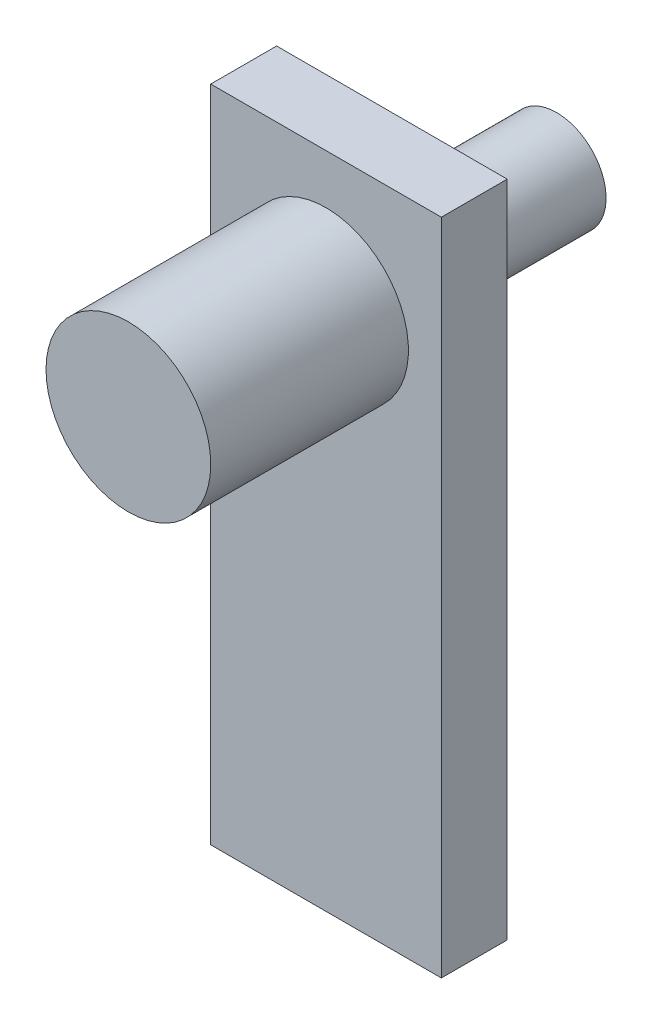
from build123d import *

# Parameters (mm, degrees)
SKETCH_1_W      = 35
SKETCH_1_H      = 100
EXTRUDE_1_DEPTH = 10
SKETCH_2_R      = 12.5
EXTRUDE_2_DEPTH = 30
SKETCH_3_R      = 7.5
EXTRUDE_3_DEPTH = 25


with BuildPart() as part:
    # 草图1 → 凸台-拉伸1 (new body)
    with BuildSketch(Plane.XY):
        Rectangle(SKETCH_1_W, SKETCH_1_H)
    extrude(amount=EXTRUDE_1_DEPTH)

    # 草图2 → 凸台-拉伸2 (add)
    with BuildSketch(Plane.XY.offset(10)):
        with Locations(Location((0, 30, 0), (0, 0, 180))):
            Circle(SKETCH_2_R)
    extrude(amount=EXTRUDE_2_DEPTH)

    # 草图3 → 凸台-拉伸3 (add)
    with BuildSketch(Plane(origin=(0, 0, 0), x_dir=(-1, 0, 0), z_dir=(0, 0, -1))):
        with Locations((0, 30)):
            Circle(SKETCH_3_R)
    extrude(amount=EXTRUDE_3_DEPTH)


solid = part.part
